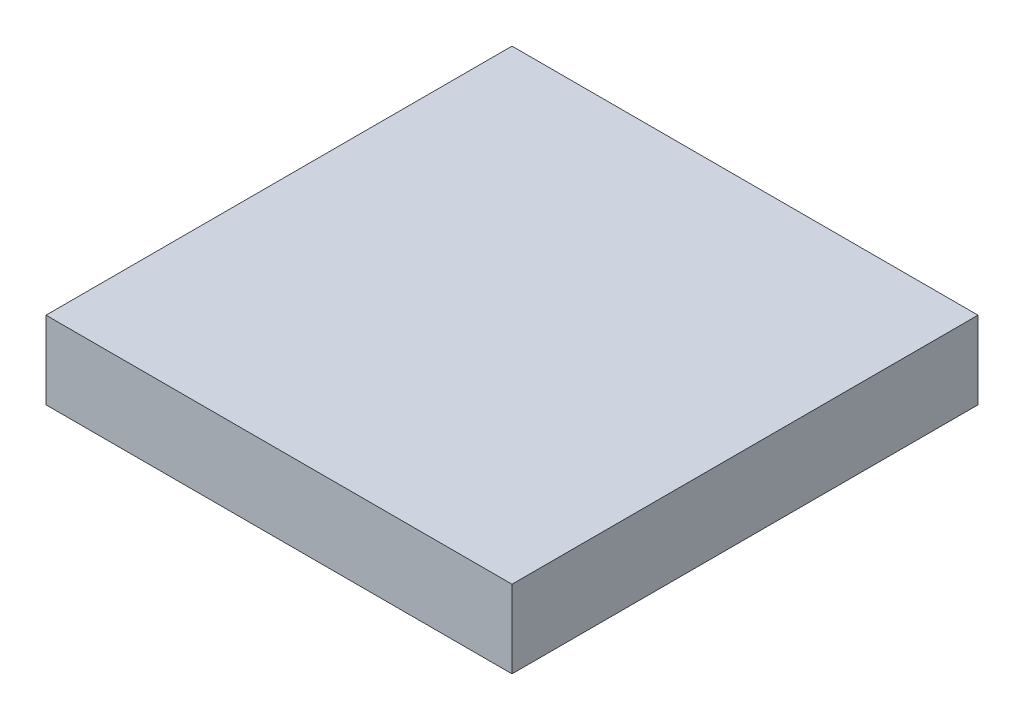
SolidWorks part; units mm, degrees
ref_plane "Front Plane" through (0, 0, 0) normal (0, 0, 1) x (1, 0, 0)
ref_plane "Top Plane" through (0, 0, 0) normal (0, 1, 0) x (1, 0, 0)
ref_plane "Right Plane" through (0, 0, 0) normal (1, 0, 0) x (0, 0, -1)
sketch "Sketch1" plane through (0, 0, 0) normal (0, 1, 0) x (1, 0, 0)
  line L1 (-60, 60) -> (60, 60)
  line L2 (-60, 60) -> (-60, -60)
  line L3 (-60, -60) -> (60, -60)
  line L4 (60, 60) -> (60, -60)
  line L5 (-60, 60) -> (60, -60) construction
  line L6 (-60, -60) -> (60, 60) construction
  point P0 (0, 0)
  dimension "D1" = 120
  dimension "D2" = 120
extrude "Boss-Extrude1" add sketch "Sketch1" along normal blind 20
